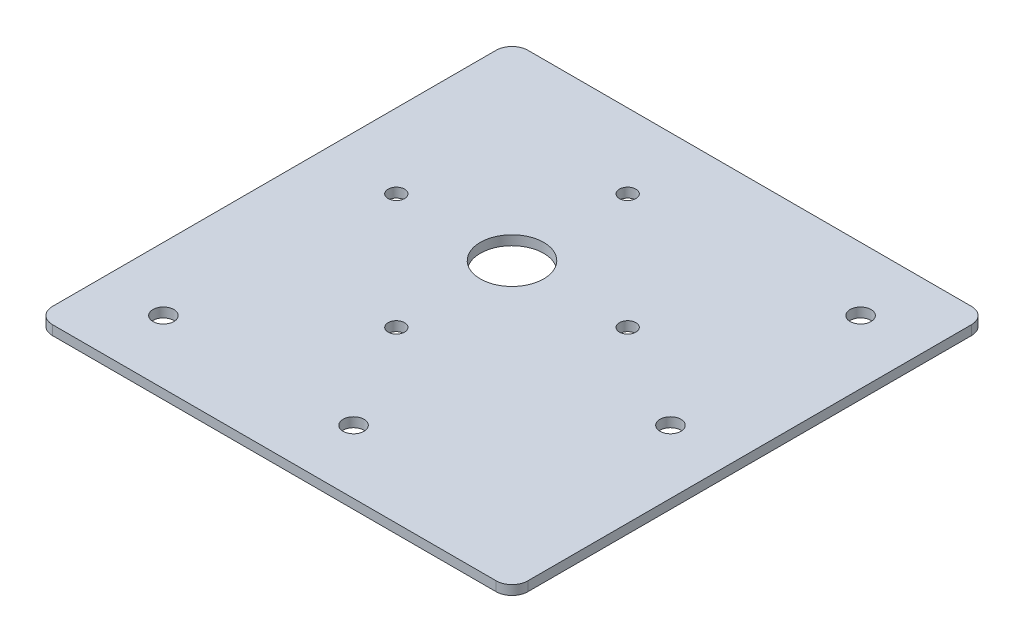
SolidWorks part; units mm, degrees
material "普通碳钢"
ref_plane "前视基准面" through (0, 0, 0) normal (0, 0, 1) x (1, 0, 0)
ref_plane "上视基准面" through (0, 0, 0) normal (0, 1, 0) x (1, 0, 0)
ref_plane "右视基准面" through (0, 0, 0) normal (1, 0, 0) x (0, 0, -1)
sketch "草图1" plane through (0, 0, 0) normal (0, 1, 0) x (1, 0, 0)
  line L1 (-75, 75) -> (75, 75)
  line L2 (-75, 75) -> (-75, -75)
  line L3 (-75, -75) -> (75, -75)
  line L4 (75, 75) -> (75, -75)
  line L5 (-75, 75) -> (75, -75) construction
  line L6 (-75, -75) -> (75, 75) construction
  point P0 (0, 0)
  dimension "D1" = 150
extrude "凸台-拉伸1" add sketch "草图1" along normal blind 3
hole_wizard "Ø6.6 (6.6) 直径孔1" positions "草图3" profile "草图2" hole size "Ø6.6" standard "ISO" end condition through all
sketch "草图3" plane through (0, 3, 0) normal (0, 1, 0) x (-1, 0, 0)
  line L0 (75, 75) -> (-75, 75) construction
  line L1 (-75, 75) -> (-75, -75) construction
  line L2 (75, -75) -> (75, 75) construction
  line L3 (-75, -75) -> (75, -75) construction
  point P0 (-55, 5)
  point P1 (-5, 55)
  point P3 (55, 55)
  point P5 (-55, -55)
  dimension "D1" = 20
  dimension "D2" = 20
  dimension "D3" = 20
  dimension "D4" = 60
  dimension "D5" = 60
  dimension "D6" = 20
sketch "草图2" plane through (55, 3, 5) normal (1, 0, 0) x (0, 0, 1)
  line L0 (0, 0) -> (0, 3)
  line L1 (0, 3) -> (3.3, 3)
  line L2 (3.3, 3) -> (3.3, 0)
  line L5 (3.3, 0) -> (0, 0)
  line L11 (0, -6.35) -> (0, 107.95) construction
  dimension "通孔孔直径" = 6.6
  dimension "通孔孔深度" = 3
fillet "圆角1" radius 5 4 edges at (-75, 1.5, 75) (-75, 1.5, -75) (75, 1.5, -75) (75, 1.5, 75)
sketch "草图4" plane through (0, 3, 0) normal (0, 1, 0) x (1, 0, 0)
  line L0 (75, -70) -> (75, 70) construction
  line L1 (-70, -75) -> (70, -75) construction
  circle A0 centre (-15, 15) radius 10
  circle A1 centre (-15, 15) radius 36.5 construction
  circle A2 centre (-15, 51.5) radius 2.6
  circle A3 centre (21.5, 15) radius 2.6
  circle A4 centre (-15, -21.5) radius 2.6
  circle A5 centre (-51.5, 15) radius 2.6
  dimension "D1" = 20
  dimension "D2" = 73
  dimension "D5" = 5.2
  dimension "D3" = 90
  dimension "D4" = 90
extrude "切除-拉伸1" cut sketch "草图4" against normal through all
